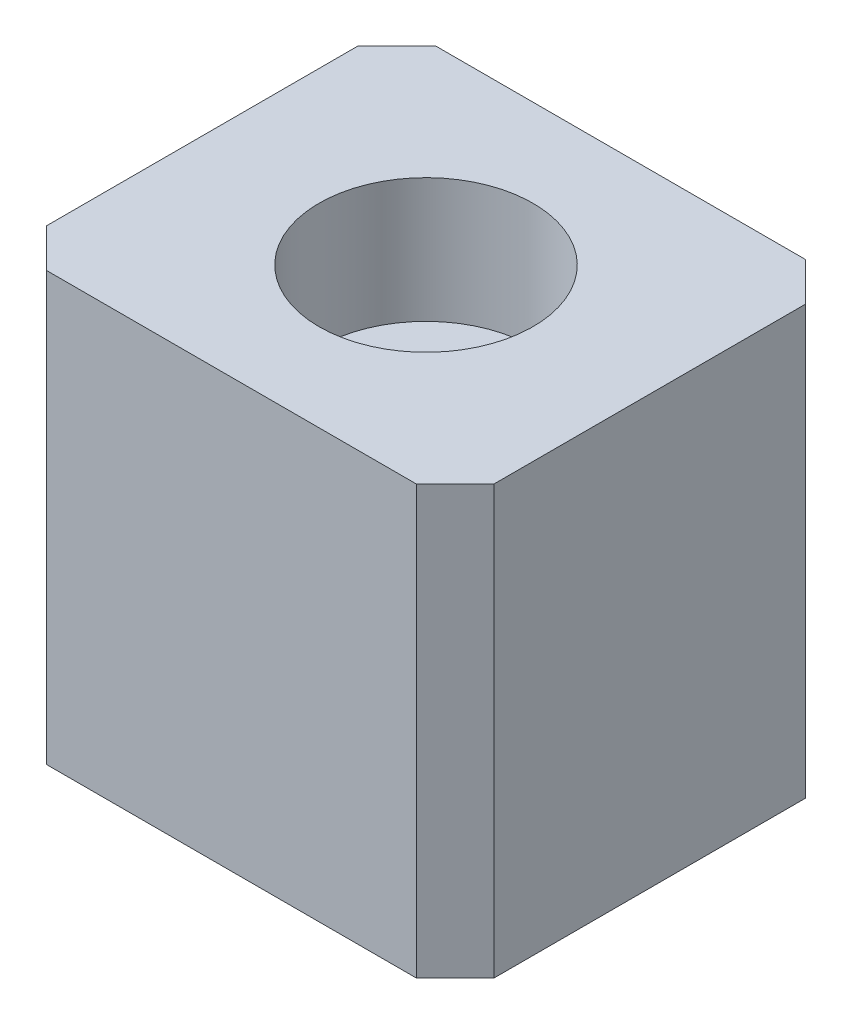
SolidWorks part; units mm, degrees
ref_plane "前视基准面" through (0, 0, 0) normal (0, 0, 1) x (1, 0, 0)
ref_plane "上视基准面" through (0, 0, 0) normal (0, 1, 0) x (1, 0, 0)
ref_plane "右视基准面" through (0, 0, 0) normal (1, 0, 0) x (0, 0, -1)
sketch "草图1" plane through (0, 0, 0) normal (0, 1, 0) x (1, 0, 0)
  line L0 (0, 10) -> (0, 0) construction
  line L1 (-11.5, 10) -> (11.5, 10)
  line L2 (-11.5, 10) -> (-11.5, -10)
  line L3 (-11.5, -10) -> (11.5, -10)
  line L4 (11.5, 10) -> (11.5, -10)
  line L5 (0, 0) -> (11.5, 0) construction
  dimension "D1" = 23
  dimension "D2" = 20
extrude "凸台-拉伸1" add sketch "草图1" along normal mid plane 22
hole_wizard "M6 六角凹头螺钉的柱形沉头孔1" positions "草图3" profile "草图2" counterbore size "M6" standard "Iso" end condition through all
sketch "草图3" plane through (0, 11, 0) normal (0, 1, 0) x (1, 0, 0)
  point P0 (0, 0)
sketch "草图2" plane through (0, 11, 0) normal (1, 0, 0) x (0, 0, 1)
  line L0 (0, 0) -> (0, 22)
  line L1 (0, 22) -> (3.3, 22)
  line L3 (3.3, 22) -> (3.3, 6.4)
  line L4 (3.3, 6.4) -> (5.5, 6.4)
  line L5 (5.5, 6.4) -> (5.5, 0)
  line L7 (5.5, 0) -> (0, 0)
  line L11 (0, -6.35) -> (0, 107.95) construction
  dimension "通孔孔直径" = 6.6
  dimension "通孔孔深度" = 22
  dimension "柱形沉头孔直径" = 11
  dimension "柱形沉头孔深度" = 6.4
chamfer "倒角1" distance 2 angle 45 4 edges at (11.5, 0, 10) (-11.5, 0, 10) (11.5, 0, -10) (-11.5, 0, -10)
